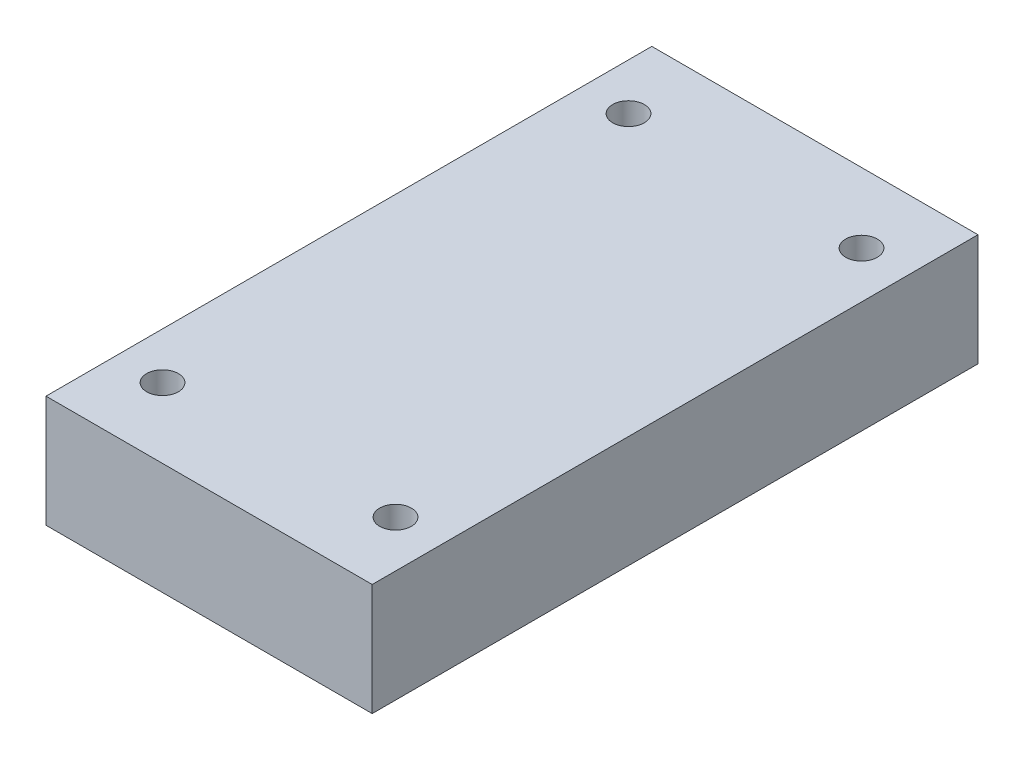
SolidWorks part; units mm, degrees
material "A3"
ref_plane "前视基准面" through (0, 0, 0) normal (0, 0, 1) x (1, 0, 0)
ref_plane "上视基准面" through (0, 0, 0) normal (0, 1, 0) x (1, 0, 0)
ref_plane "右视基准面" through (0, 0, 0) normal (1, 0, 0) x (0, 0, -1)
sketch "草图1" plane through (0, 0, 0) normal (0, 1, 0) x (1, 0, 0)
  line L1 (-35, -65) -> (35, -65)
  line L2 (-35, -65) -> (-35, 65)
  line L3 (-35, 65) -> (35, 65)
  line L4 (35, -65) -> (35, 65)
  line L5 (-35, -65) -> (35, 65) construction
  line L6 (-35, 65) -> (35, -65) construction
  point P0 (0, 0)
  dimension "D1" = 130
  dimension "D2" = 70
extrude "凸台-拉伸1" add sketch "草图1" along normal blind 24
hole_wizard "M8 螺纹孔1" positions "草图2" profile "草图3" tap size "M8" standard "GB" end condition through all
sketch "草图2" plane through (0, 24, 0) normal (0, 1, 0) x (1, 0, 0)
  line L0 (0, 65) -> (0, 0) construction
  line L1 (35, 65) -> (-35, 65) construction
  line L2 (0, 0) -> (35, 0) construction
  line L3 (35, -65) -> (35, 65) construction
  point P0 (-25, -50)
  point P14 (-25, 50)
  point P15 (25, 50)
  point P16 (25, -50)
  dimension "D1" = 50
  dimension "D2" = 100
sketch "草图3" plane through (-25, 24, 50) normal (1, 0, 0) x (0, 0, 1)
  line L0 (0, 0) -> (0, 24)
  line L1 (0, 24) -> (3.4, 24)
  line L2 (3.4, 24) -> (3.4, 0)
  line L5 (3.4, 0) -> (0, 0)
  line L11 (0, -6.35) -> (0, 107.95) construction
  dimension "通孔螺纹孔钻头直径" = 6.8
  dimension "通孔螺纹孔钻头深度" = 24
cosmetic thread "孔螺蚊线1" parameters "D2"=8
cosmetic thread "孔螺蚊线2" parameters "D2"=8
cosmetic thread "孔螺蚊线3" parameters "D2"=8
cosmetic thread "孔螺蚊线4" parameters "D2"=8
